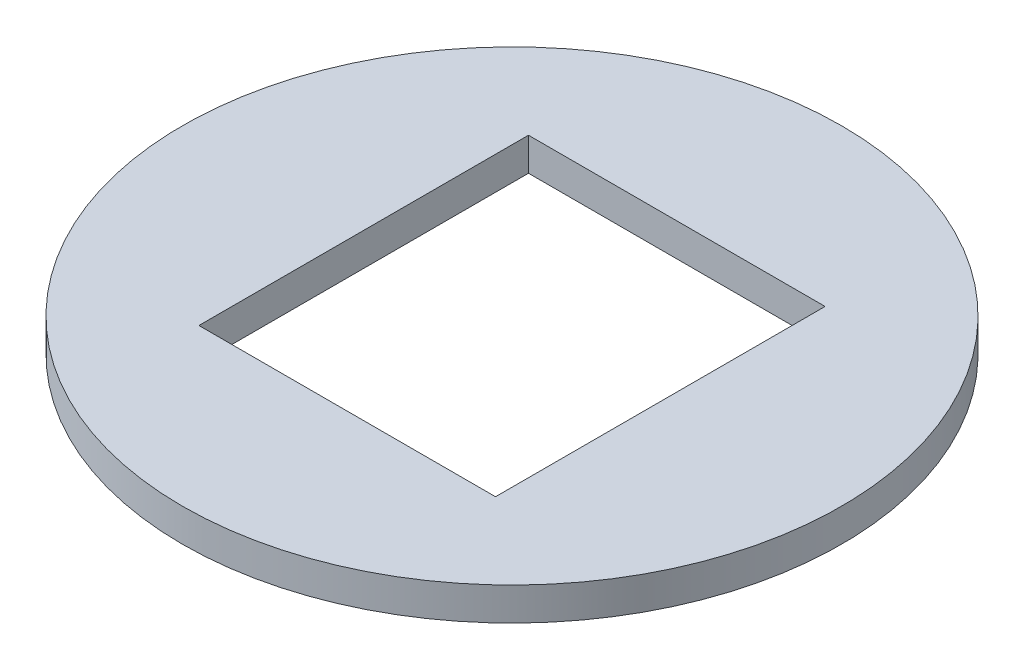
SolidWorks part; units mm, degrees
ref_plane "Front Plane" through (0, 0, 0) normal (0, 0, 1) x (1, 0, 0)
ref_plane "Top Plane" through (0, 0, 0) normal (0, 1, 0) x (1, 0, 0)
ref_plane "Right Plane" through (0, 0, 0) normal (1, 0, 0) x (0, 0, -1)
other "Configuration Table"
sketch "Sketch1" plane through (0, 0, 0) normal (0, 1, 0) x (1, 0, 0)
  circle A0 centre (0, 0) radius 500
  dimension "D1" = 1000
extrude "Boss-Extrude1" add sketch "Sketch1" along normal blind 50
sketch "Sketch2" plane through (0, 50, 0) normal (0, 1, 0) x (1, 0, 0)
  line L1 (-225, 250) -> (225, 250)
  line L2 (-225, 250) -> (-225, -250)
  line L3 (-225, -250) -> (225, -250)
  line L4 (225, 250) -> (225, -250)
  line L5 (-225, 250) -> (225, -250) construction
  line L6 (-225, -250) -> (225, 250) construction
  point P0 (0, 0)
  dimension "D1" = 450
  dimension "D2" = 500
extrude "Cut-Extrude1" cut sketch "Sketch2" against normal through all both and the other way through all
